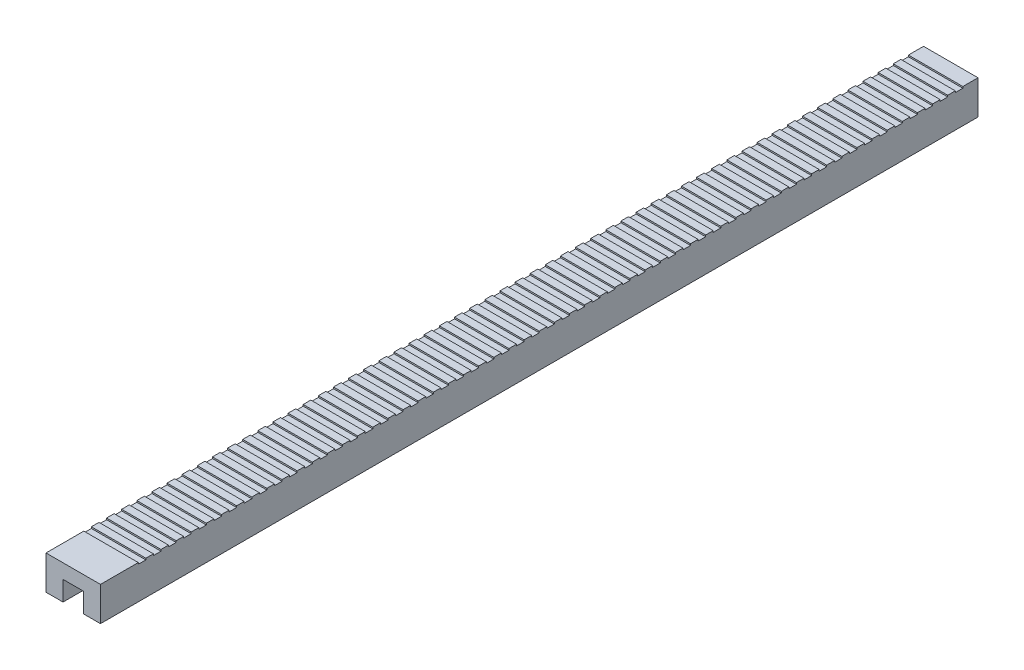
SolidWorks part; units mm, degrees
material "PE"
ref_plane "Front Plane" through (0, 0, 0) normal (0, 0, 1) x (1, 0, 0)
ref_plane "Top Plane" through (0, 0, 0) normal (0, 1, 0) x (1, 0, 0)
ref_plane "Right Plane" through (0, 0, 0) normal (1, 0, 0) x (0, 0, -1)
sketch "Sketch1" plane through (0, 0, 0) normal (0, 0, 1) x (1, 0, 0)
  line L0 (0, 22.5) -> (0, 3.5)
  line L1 (-36, 22.5) -> (36, 22.5)
  line L2 (-36, 22.5) -> (-36, -22.5)
  line L3 (-36, -22.5) -> (-13.5, -22.5)
  line L4 (36, 22.5) -> (36, -22.5)
  line L5 (-36, 22.5) -> (36, -22.5) construction
  line L6 (-36, -22.5) -> (36, 22.5) construction
  line L8 (-13.5, -22.5) -> (-13.5, 3.5)
  line L9 (-13.5, 3.5) -> (13.5, 3.5)
  line L10 (13.5, -22.5) -> (13.5, 3.5)
  line L11 (13.5, -22.5) -> (36, -22.5)
  point P0 (0, 0)
  dimension "D1" = 72
  dimension "D2" = 45
  dimension "D3" = 27
  dimension "D4" = 19
extrude "Boss-Extrude1" add sketch "Sketch1" along normal blind 1160 contours L8 L9 L0 L1 L2 L3 | L10 L11 L4 L1 L0 L9
sketch "Sketch2" plane through (0, 22.5, 0) normal (0, 1, 0) x (1, 0, 0)
  line L0 (-36, -1160) -> (-36, 0) construction
  line L1 (-36, -20) -> (36, -20)
  line L2 (-36, -20) -> (-36, -30)
  line L3 (-36, -30) -> (36, -30)
  line L4 (36, -20) -> (36, -30)
  line L5 (36, -1160) -> (36, 0) construction
  line L6 (-36, 0) -> (36, 0) construction
  dimension "D1" = 20
  dimension "D2" = 10
extrude "Cut-Extrude1" cut sketch "Sketch2" against normal blind 2
pattern_linear "LPattern1" count 55 spacing 20 along (0, 0, 1) of "Cut-Extrude1"
